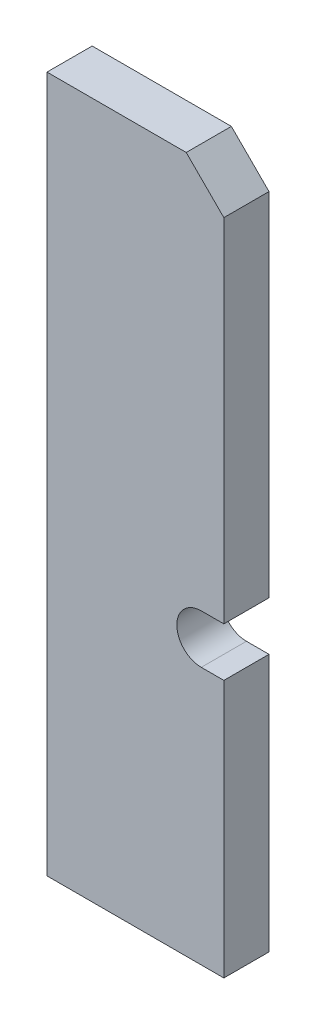
SolidWorks part; units mm, degrees
ref_plane "前视基准面" through (0, 0, 0) normal (0, 0, 1) x (1, 0, 0)
ref_plane "上视基准面" through (0, 0, 0) normal (0, 1, 0) x (1, 0, 0)
ref_plane "右视基准面" through (0, 0, 0) normal (1, 0, 0) x (0, 0, -1)
sketch "草图1" plane through (0, 0, 0) normal (0, 0, 1) x (1, 0, 0)
  line L0 (0, 0) -> (47, 0)
  line L1 (47, 0) -> (47, 185)
  line L2 (47, 185) -> (0, 185)
  line L3 (0, 185) -> (0, 0)
  dimension "D1" = 47
  dimension "D2" = 185
extrude "凸台-拉伸1" add sketch "草图1" along normal mid plane 12
sketch "草图2" plane through (0, 0, 6) normal (0, 0, 1) x (1, 0, 0)
  line L0 (0, 0) -> (47, 0) construction
  line L1 (35, 165) -> (12, 165)
  line L2 (35, 165) -> (35, 12)
  line L3 (35, 12) -> (12, 12)
  line L4 (12, 165) -> (12, 12)
  line L5 (0, 185) -> (0, 0) construction
  line L6 (47, 0) -> (47, 185) construction
  line L7 (47, 185) -> (0, 185) construction
  dimension "D1" = 12
  dimension "D2" = 12
  dimension "D3" = 12
  dimension "D4" = 20
chamfer "倒角1" distance 10 angle 45 1 edges at (47, 185, 0)
extrude "切除-拉伸1" [suppressed] cut sketch "草图2" against normal up to next
fillet "圆角1" [suppressed] radius 2
sketch "草图3" plane through (0, 0, -6) normal (0, 0, -1) x (-1, 0, 0)
  line L0 (-47, 81.5) -> (-41, 81.5)
  line L1 (-47, 0) -> (-47, 175) construction
  line L2 (-41, 68.5) -> (-47, 68.5)
  line L3 (-47, 68.5) -> (-47, 81.5)
  line L4 (0, 0) -> (-47, 0) construction
  arc A0 (-41, 81.5) -> (-41, 68.5) centre (-41, 75) cw
  dimension "D1" = 6.5
  dimension "D2" = 6
  dimension "D3" = 75
extrude "切除-拉伸2" cut sketch "草图3" against normal up to next
